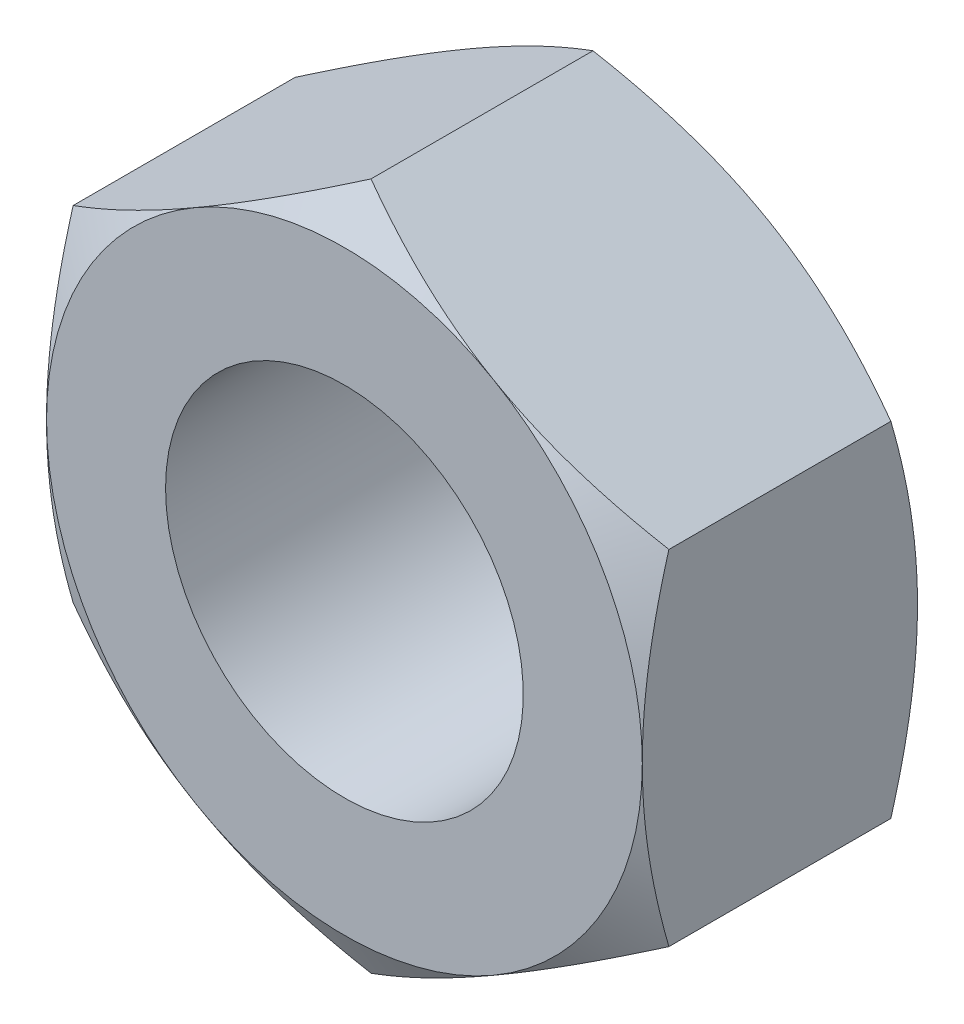
SolidWorks part; units mm, degrees
ref_plane "Front Plane" through (0, 0, 0) normal (0, 0, 1) x (1, 0, 0)
ref_plane "Top Plane" through (0, 0, 0) normal (0, 1, 0) x (1, 0, 0)
ref_plane "Right Plane" through (0, 0, 0) normal (1, 0, 0) x (0, 0, -1)
sketch "Sketch1" plane through (0, 0, 0) normal (0, 0, 1) x (1, 0, 0)
  line L1 (0, 12.5) -> (-10.8253, 6.25)
  line L2 (-10.8253, 6.25) -> (-10.8253, -6.25)
  line L3 (-10.8253, -6.25) -> (0, -12.5)
  line L4 (0, -12.5) -> (10.8253, -6.25)
  line L5 (10.8253, -6.25) -> (10.8253, 6.25)
  line L6 (10.8253, 6.25) -> (0, 12.5)
  circle A0 centre (0, 0) radius 10.8253 construction
  dimension "D1" = 25
extrude "Boss-Extrude1" add sketch "Sketch1" along normal mid plane 10
sketch "Sketch2" plane through (0, 0, 5) normal (0, 0, 1) x (1, 0, 0)
  line L0 (10.8253, 6.25) -> (0, 12.5) construction
  circle A0 centre (0, 0) radius 10.8253
extrude "Cut-Extrude1" cut sketch "Sketch2" against normal blind 10 draft 60 flip side to cut
mirror "Mirror1" about plane through (0, 0, 0) normal (0, 0, 1) of "Cut-Extrude1"
sketch "Sketch3" plane through (0, 0, -5) normal (0, 0, -1) x (-1, 0, 0)
  circle A0 centre (0, 0) radius 6.5
  dimension "D1" = 13
extrude "Cut-Extrude2" cut sketch "Sketch3" against normal blind 10
